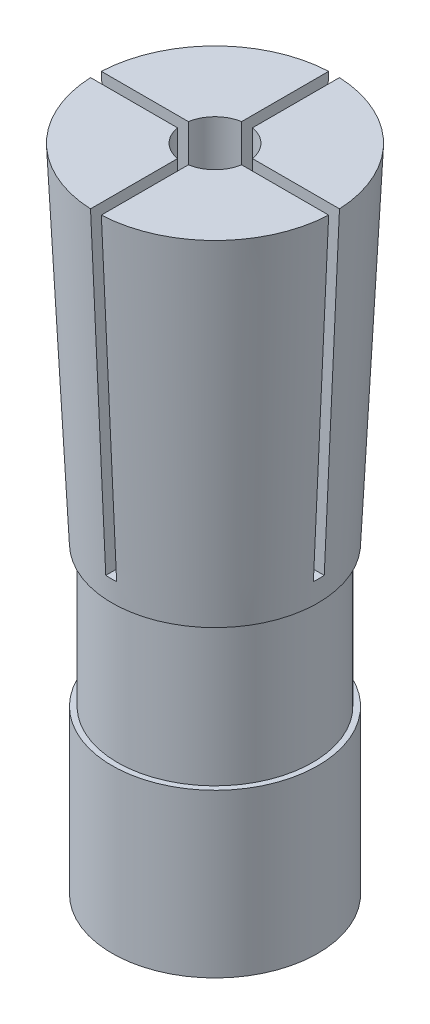
SolidWorks part; units mm, degrees
material "S45C"
ref_plane "前视基准面" through (0, 0, 0) normal (0, 0, 1) x (1, 0, 0)
ref_plane "上视基准面" through (0, 0, 0) normal (0, 1, 0) x (1, 0, 0)
ref_plane "右视基准面" through (0, 0, 0) normal (1, 0, 0) x (0, 0, -1)
sketch "草图1" plane through (0, 0, 0) normal (0, 0, 1) x (1, 0, 0)
  line L0 (0, 0) -> (0, 60) construction
  line L1 (0, 60) -> (11, 60)
  line L2 (11, 60) -> (9.5, 28)
  line L3 (9.5, 28) -> (9, 28)
  line L4 (9, 28) -> (9, 15)
  line L5 (9, 15) -> (9.5, 15)
  line L6 (9.5, 15) -> (9.5, 0)
  line L7 (9.5, 0) -> (0, 0)
  line L8 (0, 0) -> (0, 60)
  dimension "D1" = 19
  dimension "D2" = 18
  dimension "D3" = 15
  dimension "D4" = 32
  dimension "D5" = 60
  dimension "D6" = 22
revolve "旋转1" add sketch "草图1" angle 360 about L0
sketch "草图2" plane through (0, 60, 0) normal (0, 1, 0) x (1, 0, 0)
  circle A0 centre (0, 0) radius 3
  dimension "D1" = 6
extrude "切除-拉伸1" cut sketch "草图2" against normal through all
hole_wizard "M10 螺纹孔1" positions "3D草图1" profile "草图3" tap size "M10" standard "GB"
sketch3d "3D草图1"
  point P0 (0, 0, 0)
cosmetic thread "孔螺蚊线1" parameters "D1"=20, "D2"=10
sketch "草图3" plane through (0, 0, 0) normal (1, 0, 0) x (0, 0, -1)
  line L0 (0, 0) -> (0, 27.0537)
  line L1 (0, 27.0537) -> (4.25, 24.5)
  line L2 (4.25, 24.5) -> (4.25, 0)
  line L5 (4.25, 0) -> (0, 0)
  line L10 (0, 27.0537) -> (-4.25, 24.5) construction
  line L11 (0, -6.35) -> (0, 107.95) construction
  dimension "螺纹孔钻头直径" = 8.5
  dimension "螺纹孔钻头深度" = 24.5
  dimension "导头角度" = 118
sketch "草图4" plane through (0, 60, 0) normal (0, 1, 0) x (1, 0, 0)
  line L1 (-25, 0.5) -> (25, 0.5)
  line L2 (-25, 0.5) -> (-25, -0.5)
  line L3 (-25, -0.5) -> (25, -0.5)
  line L4 (25, 0.5) -> (25, -0.5)
  line L5 (-25, 0.5) -> (25, -0.5) construction
  line L6 (-25, -0.5) -> (25, 0.5) construction
  point P0 (0, 0)
  dimension "D1" = 1
  dimension "D2" = 50
extrude "切除-拉伸2" cut sketch "草图4" against normal blind 30
sketch "草图5" plane through (0, 60, 0) normal (0, 1, 0) x (1, 0, 0)
  line L1 (0.5, 25) -> (-0.5, 25)
  line L2 (0.5, 25) -> (0.5, -25)
  line L3 (0.5, -25) -> (-0.5, -25)
  line L4 (-0.5, 25) -> (-0.5, -25)
  line L5 (0.5, 25) -> (-0.5, -25) construction
  line L6 (0.5, -25) -> (-0.5, 25) construction
  point P0 (0, 0)
  dimension "D1" = 1
  dimension "D2" = 50
extrude "切除-拉伸3" cut sketch "草图5" against normal blind 30
sketch "草图6" plane through (0, 0, 0) normal (0, 0, 1) x (1, 0, 0)
  line L0 (9.5, 0) -> (10.9886, 60) construction
  line L2 (-9.5, 0) -> (-10.9217, 57.3014) construction
  line L3 (10.9886, 60) -> (0.5, 60) construction
sketch "草图7" plane through (0, 0, 0) normal (1, 0, 0) x (0, 0, -1)
  line L0 (-9.5, 0) -> (-10.9886, 60) construction
  line L1 (9.5, 0) -> (10.9886, 60) construction
